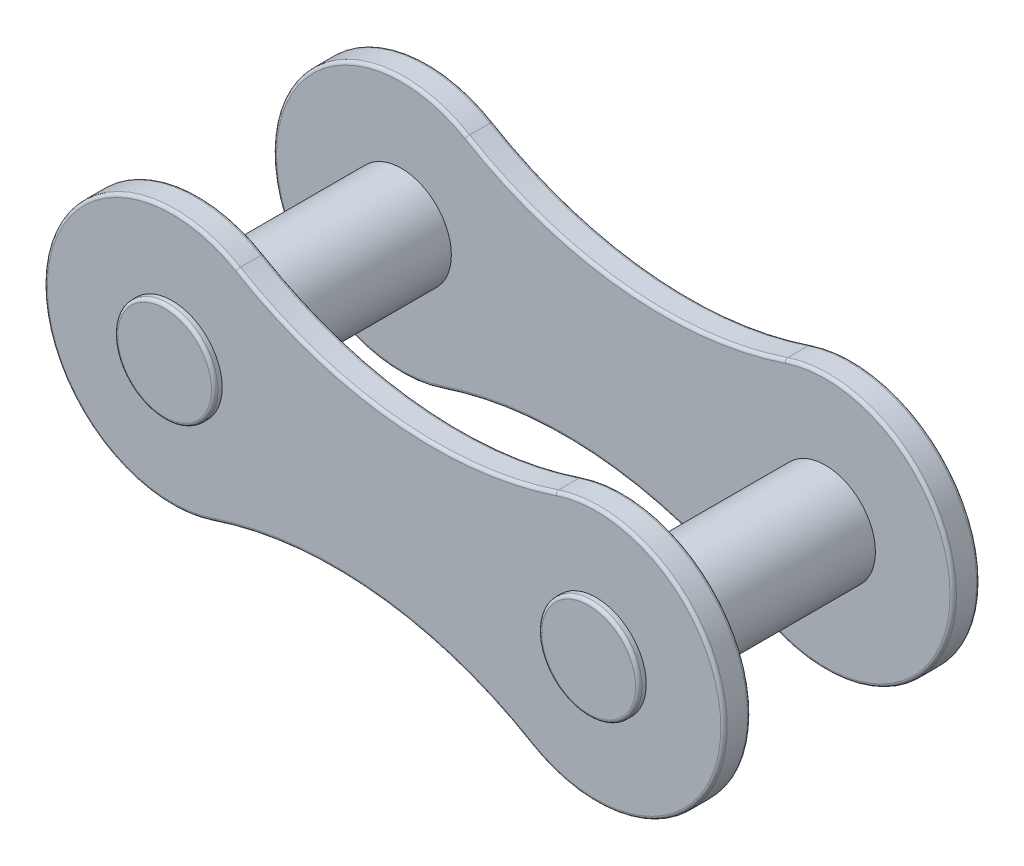
SolidWorks part; units mm, degrees
ref_plane "Front Plane" through (0, 0, 0) normal (0, 0, 1) x (1, 0, 0)
ref_plane "Top Plane" through (0, 0, 0) normal (0, 1, 0) x (1, 0, 0)
ref_plane "Right Plane" through (0, 0, 0) normal (1, 0, 0) x (0, 0, -1)
sketch "Sketch1" plane through (0, 0, 0) normal (0, 0, 1) x (1, 0, 0)
  line L2 (-120.8263, -7.992) -> (41.1869, 88.7149)
  line L3 (-31.09, -113.6198) -> (90.5295, 30.6341)
  line L4 (-139.5744, -24.2995) -> (-149.7602, -41.5113)
  line L5 (-44.6713, -126.0003) -> (-30.0489, -112.3553)
  line L6 (-30.0489, -112.3553) -> (-19.8631, -95.1434)
  line L7 (-19.8631, -95.1434) -> (-14.939, -75.7591)
  line L8 (-14.939, -75.7591) -> (-15.6756, -55.7726)
  line L9 (-15.6756, -55.7726) -> (-22.0132, -36.8033)
  line L10 (-22.0132, -36.8033) -> (-33.4383, -20.3879)
  line L11 (-33.4383, -20.3879) -> (-49.0254, -7.8562)
  line L12 (-49.0254, -7.8562) -> (-67.5117, -0.2236)
  line L13 (-67.5117, -0.2236) -> (-87.3995, 1.8917)
  line L14 (-87.3995, 1.8917) -> (-107.0777, -1.6818)
  line L15 (-107.0777, -1.6818) -> (-124.952, -10.6545)
  line L16 (-124.952, -10.6545) -> (-139.5744, -24.2995)
  line L17 (-149.7602, -41.5113) -> (-154.6843, -60.8957)
  line L18 (-154.6843, -60.8957) -> (-153.9477, -80.8821)
  line L19 (-153.9477, -80.8821) -> (-147.6101, -99.8515)
  line L20 (-147.6101, -99.8515) -> (-136.185, -116.2669)
  line L21 (-136.185, -116.2669) -> (-120.5979, -128.7985)
  line L22 (-120.5979, -128.7985) -> (-102.1116, -136.4312)
  line L23 (-102.1116, -136.4312) -> (-82.2238, -138.5465)
  line L24 (-82.2238, -138.5465) -> (-62.5456, -134.973)
  line L25 (-62.5456, -134.973) -> (-44.6713, -126.0003)
  line L27 (82.5828, 23.4986) -> (95.7099, 38.5875)
  line L28 (95.7099, 38.5875) -> (99.534, 58.2185)
  line L29 (99.534, 58.2185) -> (93.0301, 77.1315)
  line L30 (93.0301, 77.1315) -> (77.9412, 90.2587)
  line L31 (77.9412, 90.2587) -> (58.3101, 94.0827)
  line L32 (58.3101, 94.0827) -> (39.3972, 87.5789)
  line L33 (39.3972, 87.5789) -> (26.27, 72.4899)
  line L34 (26.27, 72.4899) -> (22.446, 52.8589)
  line L35 (22.446, 52.8589) -> (28.9498, 33.9459)
  line L36 (28.9498, 33.9459) -> (44.0388, 20.8187)
  line L37 (44.0388, 20.8187) -> (63.6698, 16.9947)
  line L38 (63.6698, 16.9947) -> (82.5828, 23.4986)
  arc A2 (-120.8263, -7.992) -> (-31.09, -113.6198) centre (-84.8117, -68.3274) ccw
  arc A3 (41.1869, 88.7149) -> (90.5295, 30.6341) centre (60.99, 55.5387) cw
  circle A4 centre (-84.8117, -68.3274) radius 69.5515 construction
  circle A5 centre (60.99, 55.5387) radius 37.3205 construction
  dimension "D1" = 730
  dimension "D2" = 20
  dimension "D3" = 20
sketch "Sketch2" plane through (0, 0, 0) normal (0, 0, 1) x (1, 0, 0)
  line L0 (-31.09, -113.6198) -> (90.5295, 30.6341) construction
  line L1 (-120.8263, -7.992) -> (41.1869, 88.7149) construction
  line L2 (-31.09, -113.6198) -> (90.5295, 30.6341)
  line L3 (-120.8263, -7.992) -> (41.1869, 88.7149)
  arc A0 (90.5295, 30.6341) -> (41.1869, 88.7149) centre (60.99, 55.5387) ccw construction
  arc A1 (-120.8263, -7.992) -> (-31.09, -113.6198) centre (-84.8117, -68.3274) ccw construction
  arc A2 (90.5295, 30.6341) -> (41.1869, 88.7149) centre (60.99, 55.5387) ccw
  arc A3 (-120.8263, -7.992) -> (-31.09, -113.6198) centre (-84.8117, -68.3274) ccw
  circle A4 centre (-87.3995, 1.8917) radius 2.5
  circle A5 centre (-67.5117, -0.2236) radius 2.5
  circle A6 centre (-87.3995, 1.8917) radius 6
  circle A7 centre (-67.5117, -0.2236) radius 6
  arc A8 (-84.3367, 7.051) -> (-69.4208, 5.4646) centre (-75.1481, 22.5291) ccw
  arc A9 (-85.4904, -3.7965) -> (-70.5746, -5.3829) centre (-79.7631, -20.861) cw
  dimension "D1" = 5
  dimension "D2" = 12
  dimension "D3" = 5
  dimension "D4" = 12
  dimension "D5" = 18
sketch "Sketch3" plane through (0, 0, 0) normal (0, 0, 1) x (1, 0, 0)
  circle A2 centre (-87.3995, 1.8917) radius 2.35
  circle A3 centre (-87.3995, 1.8917) radius 2.35
  circle A4 centre (-67.5117, -0.2236) radius 6 construction
  circle A5 centre (-67.5117, -0.2236) radius 2.35
  circle A6 centre (-67.5117, -0.2236) radius 2.35
  arc A7 (-70.5746, -5.3829) -> (-85.4904, -3.7965) centre (-79.7631, -20.861) ccw construction
  arc A8 (-84.3367, 7.051) -> (-69.4208, 5.4646) centre (-75.1481, 22.5291) ccw construction
  circle A9 centre (-87.3995, 1.8917) radius 6 construction
  arc A10 (-70.5746, -5.3829) -> (-69.4208, 5.4646) centre (-67.5117, -0.2236) ccw
  arc A11 (-70.5746, -5.3829) -> (-85.4904, -3.7965) centre (-79.7631, -20.861) ccw
  arc A12 (-84.3367, 7.051) -> (-69.4208, 5.4646) centre (-75.1481, 22.5291) ccw
  arc A13 (-84.3367, 7.051) -> (-85.4904, -3.7965) centre (-87.3995, 1.8917) ccw
  dimension "D1" = 0.15
  dimension "D2" = 0.15
extrude "Boss-Extrude1" add sketch "Sketch3" along normal blind 1.25 from offset 4.75
mirror "Mirror1" about plane through (0, 0, 0) normal (0, 0, 1) of bodies 111
sketch "Sketch4" plane through (0, 0, 0) normal (0, 0, 1) x (1, 0, 0)
  circle A0 centre (-67.5117, -0.2236) radius 2.35 construction
  circle A1 centre (-87.3995, 1.8917) radius 2.35 construction
  circle A2 centre (-67.5117, -0.2236) radius 2.35
  circle A3 centre (-87.3995, 1.8917) radius 2.35
extrude "Boss-Extrude2" add sketch "Sketch4" along normal blind 6.35 and the other way blind 6.35
fillet "Fillet1" radius 0.15 20 edges at (-61.5454, -0.8582, 6) (-77.8594, -2.962, 6) (-93.3659, 2.5263, 6) (-61.5454, -0.8582, 4.75) (-77.8594, -2.962, 4.75) (-93.3659, 2.5263, 4.75) (-61.5454, -0.8582, -6) (-77.8594, -2.962, -6) (-93.3659, 2.5263, -6) (-61.5454, -0.8582, -4.75) (-77.8594, -2.962, -4.75) (-93.3659, 2.5263, -4.75) (-85.0495, 1.8917, -6.35) (-65.1617, -0.2236, -6.35) (-65.1617, -0.2236, 6.35) (-85.0495, 1.8917, 6.35) (-77.0519, 4.6301, 6) (-77.0519, 4.6301, 4.75) (-77.0519, 4.6301, -6) (-77.0519, 4.6301, -4.75)
ref_plane "Plane1" through (0, 0, 0) normal (0, 0, 1) x (1, 0, 0)
sketch "Sketch5" plane through (0, 0, 0) normal (0, 0, 1) x (1, 0, 0)
  circle A0 centre (-67.5117, -0.2236) radius 2.5 construction
  circle A1 centre (-87.3995, 1.8917) radius 2.5 construction
  circle A2 centre (-67.5117, -0.2236) radius 2.5
  circle A3 centre (-87.3995, 1.8917) radius 2.5
scale "Scale1" scale about centroid uniform scaling yes scale factor 0.5
scale "Scale2" scale about centroid uniform scaling yes scale factor 0.5
scale "Scale3" scale about centroid uniform scaling yes scale factor 0.5
sketch "Sketch6" plane through (0, 0, 0) normal (0, 0, 1) x (1, 0, 0)
  line L0 (-78.6986, 0.9663) -> (-76.2126, 0.7018)
